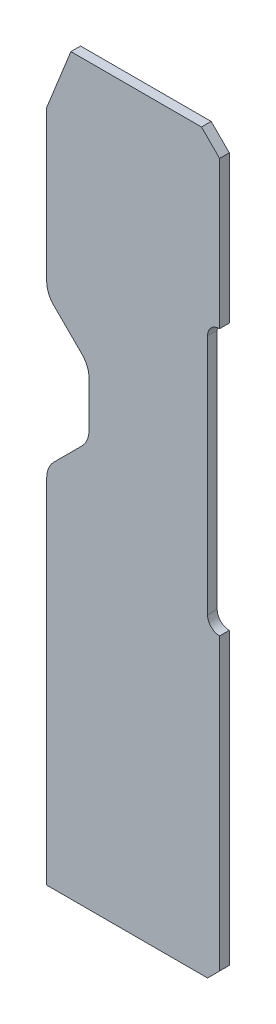
SolidWorks part; units mm, degrees
material "Q345B"
ref_plane "Front Plane" through (0, 0, 0) normal (0, 0, 1) x (1, 0, 0)
ref_plane "Top Plane" through (0, 0, 0) normal (0, 1, 0) x (1, 0, 0)
ref_plane "Right Plane" through (0, 0, 0) normal (1, 0, 0) x (0, 0, -1)
sketch "Sketch1" plane through (0, 0, 0) normal (0, 0, 1) x (1, 0, 0)
  line L0 (0, 0) -> (0, 291.7157)
  line L1 (5.8579, 305.8579) -> (29.1421, 329.1421)
  line L2 (35, 343.2843) -> (35, 380.7157)
  line L3 (29.1421, 394.8579) -> (5.8579, 418.1421)
  line L4 (0, 432.2843) -> (0, 557)
  line L5 (0, 557) -> (20, 607)
  line L6 (20, 607) -> (128, 607)
  line L7 (128, 607) -> (143, 592)
  line L8 (143, 592) -> (143, 470)
  line L10 (133, 460) -> (133, 260)
  line L12 (143, 250) -> (143, 10)
  line L13 (133, 0) -> (0, 0)
  line L14 (143, 10) -> (133, 0)
  arc A0 (143, 470) -> (133, 460) centre (143, 460) ccw
  arc A1 (143, 250) -> (133, 260) centre (143, 260) cw
  arc A2 (5.8579, 418.1421) -> (0, 432.2843) centre (20, 432.2843) cw
  arc A3 (35, 380.7157) -> (29.1421, 394.8579) centre (15, 380.7157) ccw
  arc A4 (29.1421, 329.1421) -> (35, 343.2843) centre (15, 343.2843) ccw
  arc A5 (0, 291.7157) -> (5.8579, 305.8579) centre (20, 291.7157) cw
  point P15 (143, 0)
  point P21 (135.9289, 467.0711)
  point P23 (0, 424)
  point P26 (35, 389)
  point P29 (35, 335)
  point P32 (0, 300)
  dimension "D16" = 10
  dimension "D6" = 20
  dimension "D1" = 143
  dimension "D2" = 143
  dimension "D3" = 607
  dimension "D4" = 220
  dimension "D5" = 10
  dimension "D7" = 15
  dimension "D8" = 15
  dimension "D9" = 50
  dimension "D10" = 20
  dimension "D11" = 35
  dimension "D12" = 54
  dimension "D13" = 35
  dimension "D14" = 300
  dimension "D15" = 10
extrude "Boss-Extrude1" add sketch "Sketch1" along normal blind 8
